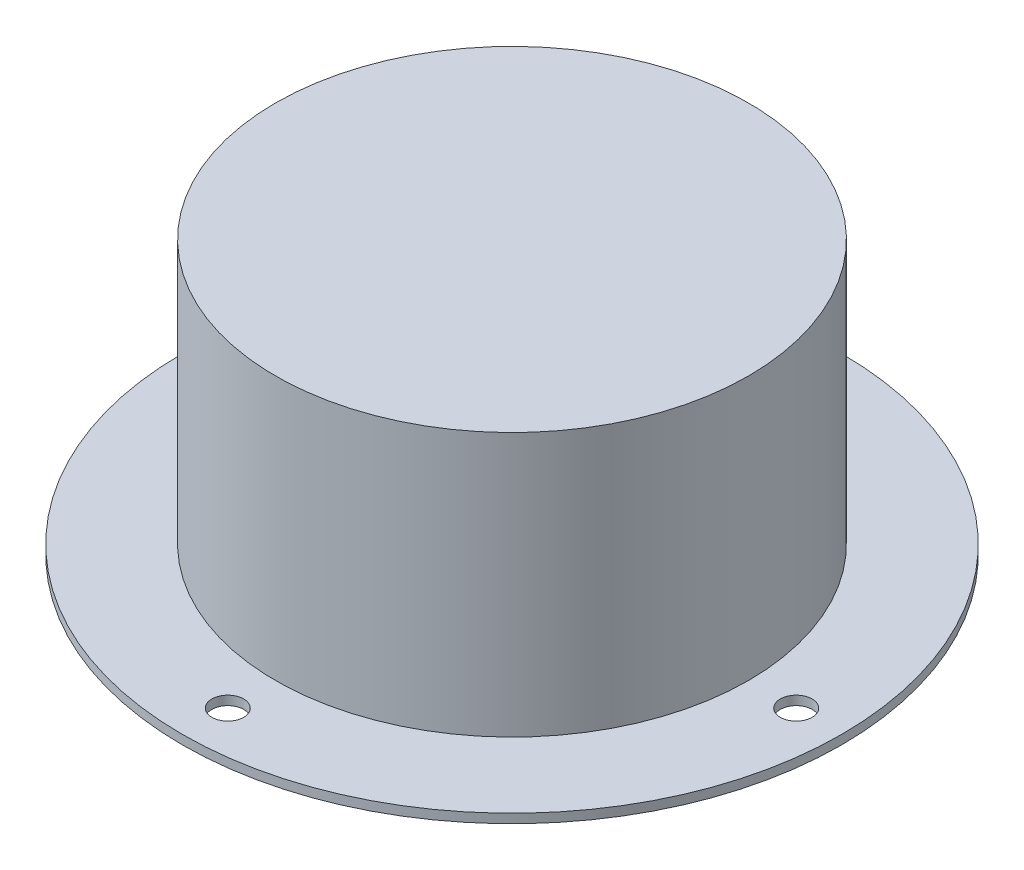
SolidWorks part; units mm, degrees
material "Q235-A"
ref_plane "Front Plane" through (0, 0, 0) normal (0, 0, 1) x (1, 0, 0)
ref_plane "Top Plane" through (0, 0, 0) normal (0, 1, 0) x (1, 0, 0)
ref_plane "Right Plane" through (0, 0, 0) normal (1, 0, 0) x (0, 0, -1)
sketch "Sketch1" plane through (0, 0, 0) normal (0, 0, 1) x (1, 0, 0)
  line L0 (-50, 0) -> (-72.5, 0)
  line L1 (-72.5, 0) -> (-72.5, 2)
  line L2 (-72.5, 2) -> (-52, 2)
  line L3 (-52, 2) -> (-52, 60)
  line L4 (-52, 60) -> (0, 60)
  line L5 (0, 60) -> (0, 58)
  line L6 (0, 58) -> (-50, 58)
  line L7 (-50, 58) -> (-50, 0)
  dimension "D1" = 72.5
  dimension "D2" = 60
  dimension "D3" = 2
  dimension "D4" = 2
  dimension "D5" = 2
  dimension "D6" = 50
revolve "Revolve1" add sketch "Sketch1" angle 360 about L5
sketch "Sketch2" plane through (0, 2, 0) normal (0, 1, 0) x (1, 0, 0)
  circle A0 centre (0, 62.5) radius 3.5
  dimension "D1" = 7
  dimension "D2" = 62.5
extrude "Cut-Extrude1" cut sketch "Sketch2" against normal through all
pattern_circular "CirPattern1" count 4 over 360 about axis through (0, 0, 0) along (0, 1, 0) of "Cut-Extrude1"
